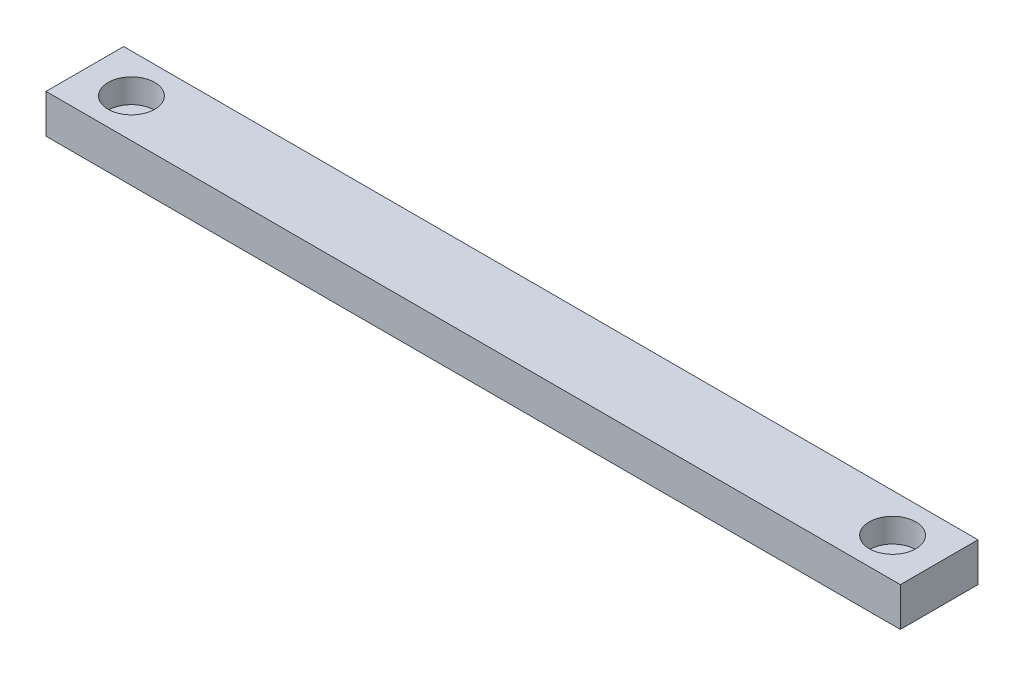
from build123d import *

# Parameters (mm, degrees)
SKETCH1_W           = 110
SKETCH1_H           = 10
BOSS_EXTRUDE1_DEPTH = 5
SKETCH2_R           = 3
CUT_EXTRUDE1_DEPTH  = 3.1


with BuildPart() as part:
    # Sketch1 → Boss-Extrude1 (new body)
    with BuildSketch(Plane(origin=(0, 0, 0), x_dir=(1, 0, 0), z_dir=(0, 1, 0))):
        Rectangle(SKETCH1_W, SKETCH1_H)
    extrude(amount=BOSS_EXTRUDE1_DEPTH)

    # Sketch2 → Cut-Extrude1 (cut)
    with BuildSketch(Plane(origin=(0, 5, 0), x_dir=(1, 0, 0), z_dir=(0, 1, 0))):
        with Locations(Location((-49, 0, 0), (0, 0, 270))):
            Circle(SKETCH2_R)
        with Locations(Location((49, 0, 0), (0, 0, 270))):
            Circle(SKETCH2_R)
    extrude(amount=-CUT_EXTRUDE1_DEPTH, mode=Mode.SUBTRACT)


solid = part.part
